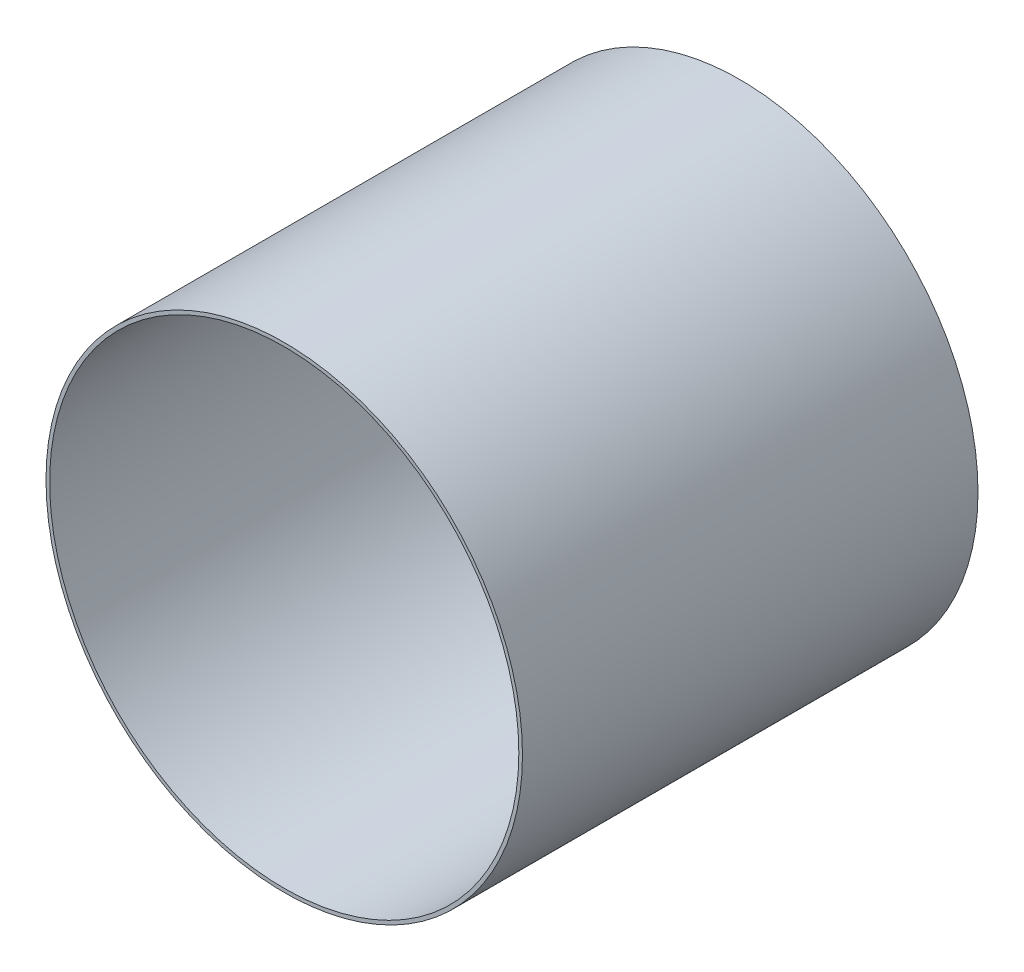
SolidWorks part; units mm, degrees
material "Q235"
ref_plane "Front Plane" through (0, 0, 0) normal (0, 0, 1) x (1, 0, 0)
ref_plane "Top Plane" through (0, 0, 0) normal (0, 1, 0) x (1, 0, 0)
ref_plane "Right Plane" through (0, 0, 0) normal (1, 0, 0) x (0, 0, -1)
sketch "Sketch1" plane through (0, 0, 0) normal (0, 0, 1) x (1, 0, 0)
  circle A0 centre (0, 0) radius 515
  dimension "D1" = 1030
extrude "Extrude-Thin1" add sketch "Sketch1" along normal mid plane 1000 thin
